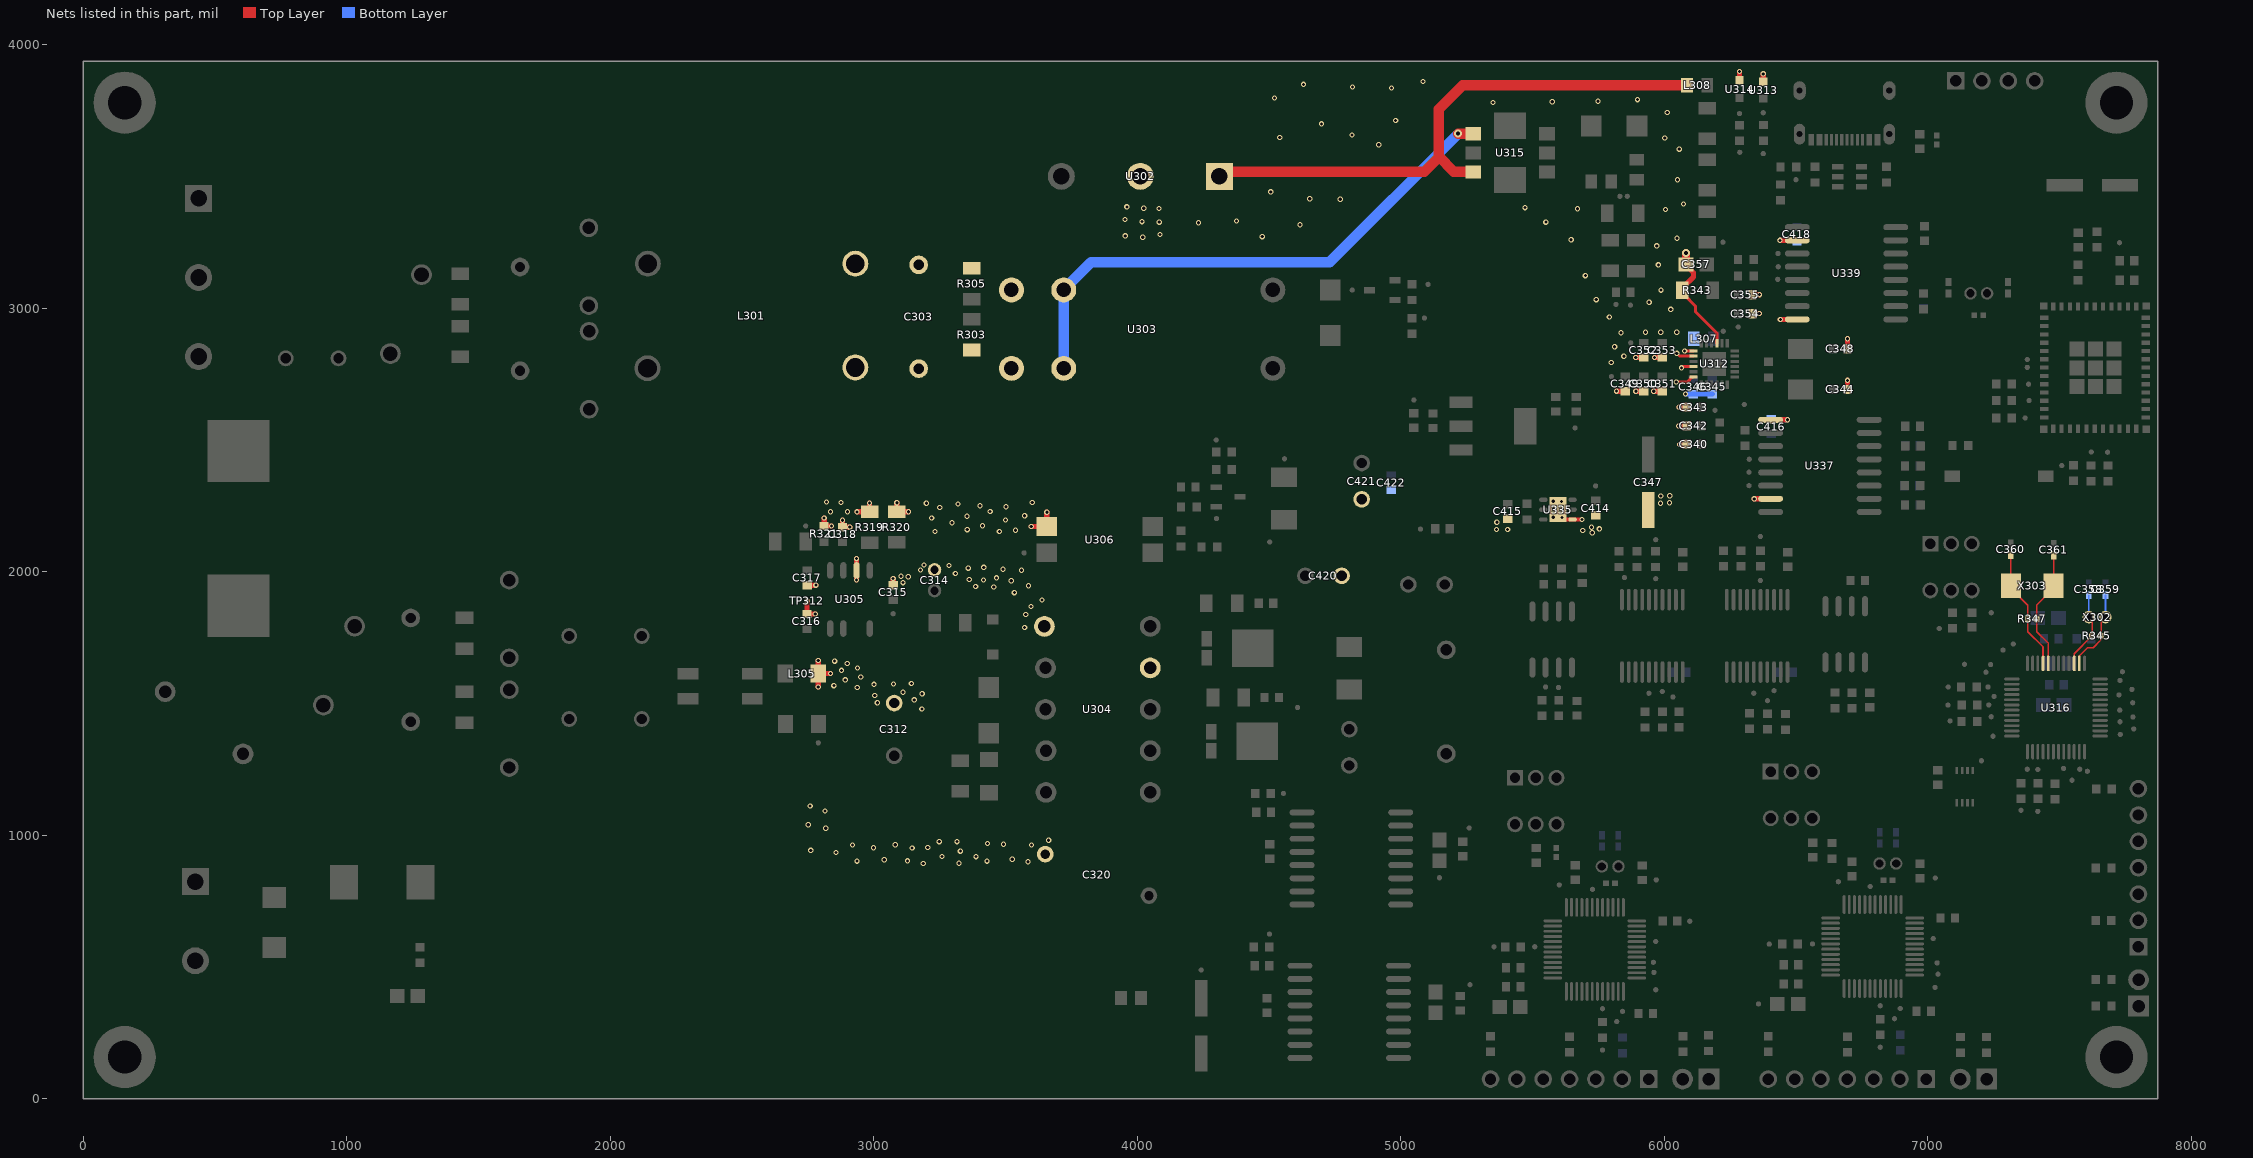
[diagram p0: the nets of this part, all layers, seen from the top]
# Altium PCB MISC84429.PcbDoc (part 2 of 5)
Units mil, origin at the board's own origin, x right, y up, seen from the top; angles counter-clockwise.
Board outline 7874.02 x 3937.01 mil, 4 copper layers (Top Layer, GND, POWER, Bottom Layer); 424 components, 202 nets, 1144 pads, 784 vias.

## Footprints (in the part's own frame and the unit in brackets; to place one, negate y for a bottom-side part, rotate by r counter-clockwise, add the part's x,y. Pads: shape width x height; smd on the part's side, far side on the other; paste and mask are expansions set on the pad) (continued)
CAP-TH_BD10.0-P5.00-D1.0-FD [mm]
  round 1.6 hole 1: 1(-2.54,0) 2(2.54,0)
  silkscreen extent -5,-5 5.08,5
CAP-TH_L7.0-W4.0-P10.00-D0.6 [mm]
  round 1.8 hole 1.1: 1(-5,0) 2(5,0)
  silkscreen extent -3.5,-2 3.5,2
CAP-TH_L8.0-W4.0-P7.50-D1.2 [mm]
  round 1.8 hole 1.2: 1(-3.75,0) 2(3.75,0)
  silkscreen extent -4,-2 4,2
CAP-TH_L10.0-W4.5-P10.00-D0.6-S4.0 [mm]
  round 1.6 hole 0.9: 1(-5,2) 2(5,-2)
  silkscreen extent -5,-2.25 5,2.25
CAP-TH_L13.0-W6.0-P10.00-D0.6 [mm]
  round 1.8 hole 1: 1(-5,0) 2(5,0)
  silkscreen extent -6.5,-3 6.5,3
CONN-TH_2P-P7.62_L15.2-W16.7-EX4.2 [mm]
  rect 2.6x2.6 hole 1.6: 1(-3.81,0)
  round 2.6 hole 1.6: 2(3.81,0)
  silkscreen extent -8.22,-10.65 8.38,4.55
CONN-TH_3P-P7.62_L15.2-W24.4-EX4.2 [mm]
  rect 2.6x2.6 hole 1.6: 1(-7.62,0)
  round 2.6 hole 1.6: 2(0,0) 3(7.62,0)
  silkscreen extent -12.03,-11 12.27,4.2
CRYSTAL-SMD_2P-L5.0-W3.2 [mm]
  rect 1.9x2.4 smd: 1(-1.95,0) 2(1.95,0)
  silkscreen extent -3.1,-1.75 3.1,1.75
CRYSTAL-SMD_L5.0-W3.2 [mm]
  rect 1.9x2.4 smd: 1(-2.05,0) 2(2.05,0)
  silkscreen extent -3.32,-1.85 3.33,1.85
F0603 [mil]
  rect 31.75x34.02 smd paste-3937.01 mask+2: 1(-29.66,0) 2(29.66,0)
  silkscreen extent -55,-25 55,25
FILTER-TH_FC-DLFW2015-5MH-20A-LF [mm]
  round 2.5 hole 1.8 paste+0 mask+0.05: 1(-5.04,-9.983) 2(5.04,-10.016) 3(4.96,10.016) 4(-5.04,10.016)
  silkscreen extent -13.72,-11.98 11.96,12.02
FUSE-SMD_L20.0-W5.0 [mm]
  rect 6x6 smd: 1(-7.45,0) 2(7.45,0)
  silkscreen extent -4.22,-2.58 4.17,2.55
FUSE-TH_L8.4-W4.0-P5.08-D0.6 [mil]
  round 60 hole 39.37 paste+0 mask+1.97: 1(-100,0) 2(100,0)
  silkscreen extent -170,-80 165,85
HDR-TH_2P-P2.54-V-M [mm]
  rect 2x2 hole 1.2: 1(-1.27,0)
  round 2 hole 1.2: 2(1.27,0)
  silkscreen extent -2.54,-1.27 2.54,1.27
HDR-TH_4P-P2.54-V-M [mm]
  rect 1.7x1.7 hole 1.1: 1(-3.81,0)
  round 1.7 hole 1.1: 2(-1.27,0) 3(1.27,0) 4(3.81,0)
  silkscreen extent -5.08,-1.27 5.08,1.27
HDR-TH_7P-P2.54-V-M [mm]
  rect 1.7x1.7 hole 1.1: 1(-7.62,0)
  round 1.7 hole 1.1: 2(-5.08,0) 3(-2.54,0) 4(0,0) 5(2.54,0) 6(5.08,0) 7(7.62,0)
  silkscreen extent -8.89,-1.25 8.89,1.25
IND-SMD_L5.4-W5.2_FXL0530 [mm]
  rect 1.9x2.5 smd: 1(-2.05,0) 2(2.05,0)
  silkscreen extent -2.7,-2.6 2.7,2.6
IND-TH_4P-L14.0-W12.0_DLSF1010-12MH-L-S [mm]
  round 1.524 hole 1 paste+0 mask+0.05: 1(-4,-3.5) 2(-4,3.5) 3(4,3.5) 4(4,-3.5)
  silkscreen extent -7.11,-5.97 6.98,6.1
L0805 [mil]
  rect 44.59x54.21 smd paste-3937.01 mask+2: 1(-38.04,0) 2(38.04,0)
  silkscreen extent -77,-40 73,40
L1206 [mm]
  rect 1.485x1.728 smd paste-100 mask+0.051: 1(-1.593,0) 2(1.593,0)
  silkscreen extent -2.56,-1.09 2.56,1.09
LED0603-R-FD [mm]
  rect 0.8x0.8 smd: 1(0.851,0) 2(-0.851,0)
  silkscreen extent -1.82,-0.86 1.77,0.86
LED0603-RD_GREEN [mm]
  rect 0.8x0.8 smd: 1(-0.799,-0.003) 2(0.799,0.003)
  silkscreen extent -1.49,-0.75 1.39,0.76
LQFP-48_L7.0-W7.0-P0.50-LS9.0-BL [mm]
  oval 0.27x1.5 smd paste+0 mask+0.05: 1(-2.75,-4.25) 2(-2.25,-4.25) 3(-1.75,-4.25) 4(-1.25,-4.25) 5(-0.75,-4.25) 6(-0.25,-4.25) 7(0.25,-4.25) 8(0.75,-4.25) 9(1.25,-4.25) 10(1.75,-4.25) 11(2.25,-4.25) 12(2.75,-4.25) 25(2.75,4.25) 26(2.25,4.25) 27(1.75,4.25) 28(1.25,4.25) 29(0.75,4.25) 30(0.25,4.25) 31(-0.25,4.25) 32(-0.75,4.25) 33(-1.25,4.25) 34(-1.75,4.25) 35(-2.25,4.25) 36(-2.75,4.25)
  oval 1.5x0.27 smd paste+0 mask+0.05: 13(4.25,-2.75) 14(4.25,-2.25) 15(4.25,-1.75) 16(4.25,-1.25) 17(4.25,-0.75) 18(4.25,-0.25) 19(4.25,0.25) 20(4.25,0.75) 21(4.25,1.25) 22(4.25,1.75) 23(4.25,2.25) 24(4.25,2.75) 37(-4.25,2.75) 38(-4.25,2.25) 39(-4.25,1.75) 40(-4.25,1.25) 41(-4.25,0.75) 42(-4.25,0.25) 43(-4.25,-0.25) 44(-4.25,-0.75) 45(-4.25,-1.25) 46(-4.25,-1.75) 47(-4.25,-2.25) 48(-4.25,-2.75)
  silkscreen extent -3.59,-4.46 3.3,3.34
LQFP-48_L7.0-W7.0-P0.50-LS9.0-TL [mm]
  oval 1.8x0.28 smd: 1(-4.05,2.75) 2(-4.05,2.25) 3(-4.05,1.75) 4(-4.05,1.25) 5(-4.05,0.75) 6(-4.05,0.25) 7(-4.05,-0.25) 8(-4.05,-0.75) 9(-4.05,-1.25) 10(-4.05,-1.75) 11(-4.05,-2.25) 12(-4.05,-2.75) 25(4.05,-2.75) 26(4.05,-2.25) 27(4.05,-1.75) 28(4.05,-1.25) 29(4.05,-0.75) 30(4.05,-0.25) 31(4.05,0.25) 32(4.05,0.75) 33(4.05,1.25) 34(4.05,1.75) 35(4.05,2.25) 36(4.05,2.75)
  oval 0.28x1.8 smd: 13(-2.75,-4.05) 14(-2.25,-4.05) 15(-1.75,-4.05) 16(-1.25,-4.05) 17(-0.75,-4.05) 18(-0.25,-4.05) 19(0.25,-4.05) 20(0.75,-4.05) 21(1.25,-4.05) 22(1.75,-4.05) 23(2.25,-4.05) 24(2.75,-4.05) 37(2.75,4.05) 38(2.25,4.05) 39(1.75,4.05) 40(1.25,4.05) 41(0.75,4.05) 42(0.25,4.05) 43(-0.25,4.05) 44(-0.75,4.05) 45(-1.25,4.05) 46(-1.75,4.05) 47(-2.25,4.05) 48(-2.75,4.05)
  silkscreen extent -4.42,-2.75 2.75,3.6
MBS_L4.7-W3.8-P2.40-LS7.0-TL [mm]
  rect 2x1.1 smd: 1(-3.1,1.2) 2(-3.1,-1.2) 3(3.1,-1.2) 4(3.1,1.2)
  silkscreen extent -3.23,-2.5 2.1,2.5
OSC-TH_BD3.1-P0.8-D0.3 [mm]
  round 1.2 hole 0.8: 1(0,0.8) 2(0,-0.8)
  silkscreen extent -10,-1.5 -0.7,1.5
R0402 [mm]
  rect 0.566x0.54 smd paste-100 mask+0.051: 1(-0.433,0) 2(0.433,0)
  silkscreen extent -0.94,-0.5 0.94,0.5
R0603 [mil]
  rect 31.75x34.02 smd paste-3937.01 mask+2: 1(-29.66,0) 2(29.66,0)
  silkscreen extent -55,-26 55,26
R1206 [mil]
  rect 47.54x66.97 smd paste-3937.01 mask+2: 1(-58.22,0) 2(58.22,0)
  silkscreen extent -91,-42 91,42
RELAY-TH_HF115F-XXX-1HS3 [mm]
  round 2.4 hole 1.4 paste+0 mask+0.05: 1(-12.6,3.78) 2(-12.6,-3.78) 5(7.56,3.78) 6(7.56,-3.78) 7(12.6,3.78) 8(12.6,-3.78)
  silkscreen extent -15.24,-6.35 13.84,6.35
RES-TH_L16.5-W5.6-P7.50-D1.2-S3.00 [mm]
  round 2 hole 1.4: 1(-3.8,1.5) 2(3.8,-1.5)
  silkscreen extent -8.25,-2.8 8.25,2.8
RES-TH_L17.5-W6.0-P7.50-D0.8-S7.50 [mm]
  round 2 hole 1.2 paste+0 mask+0.05: 1(-3.749,3) 2(3.749,-3)
  silkscreen extent -8.75,-3 8.75,3
SENSOR-TH_PA1005.100NL [mm]
  rect 1.27x1.52 smd: 1(1.85,3.555) 2(0,3.555) 3(-1.85,3.555) 4(-1.85,-3.555) 5(0,-3.555) 6(1.85,-3.555)
  rect 2.54x3.05 smd: 7(-2.615,0) 8(2.615,0)
  silkscreen extent -3.61,-4.19 3.6,4.19
SMA_L4.3-W2.6-LS5.2-RD [mm]
  rect 2x2 smd: 1(-2.2,0) 2(2.2,0)
  silkscreen extent -2.98,-1.5 2.6,1.5
SMB_L4.6-W3.6-LS5.4-RD [mil]
  rect 80.61x88.23 smd: 1(-95,0) 2(95,0)
  silkscreen extent -100,-77 88,77
SMC_L6.9-W5.9-LS7.9-RD [mm]
  rect 2.7x3.3 smd: 1(-3.686,0) 2(3.686,0)
  silkscreen extent -4.36,-3.1 3.98,3.1
SOD-123_L2.8-W1.8-LS3.7-RD [mm]
  rect 0.95x1.15 smd: 1(-1.692,0) 2(1.692,0)
  silkscreen extent -1.58,-0.87 1.41,0.87
SOIC-8_7P-L4.9-W3.9-P1.27-LS6.0-BL-PE3 [mm]
  oval 0.6x1.6 smd: 1(-1.905,-2.8) 2(-0.635,-2.8) 4(1.905,-2.8) 5(1.905,2.8) 6(0.635,2.8) 7(-0.635,2.8) 8(-1.905,2.8)
  silkscreen extent -2.54,-1.78 2.46,1.78
SOIC-8_L5.0-W4.0-P1.27-LS6.1-BL [mil]
  oval 22.38x76.78 smd: 1(-75,-106.5) 2(-25,-106.5) 3(25,-106.5) 4(75,-106.5) 5(75,106.5) 6(25,106.5) 7(-25,106.5) 8(-75,106.5)
  silkscreen extent -98,-58 98,58
SOIC-16_L10.3-W7.5-P1.27-LS10.3-BL [mil]
  oval 22.6x94.51 smd: 1(-175,-187.02) 2(-125,-187.02) 3(-75,-187.02) 4(-25,-187.02) 5(25,-187.02) 6(75,-187.02) 7(125,-187.02) 8(175,-187.02) 9(175,187.02) 10(125,187.02) 11(75,187.02) 12(25,187.02) 13(-25,187.02) 14(-75,187.02) 15(-125,187.02) 16(-175,187.02)
  silkscreen extent -210,-193 206,131
SOP-4_L6.5-W4.6-P2.54-LS10.2-TL [mm]
  rect 2x1.8 smd: 1(-5.1,1.27) 2(-5.1,-1.27) 3(5.1,-1.27) 4(5.1,1.27)
  silkscreen extent -4.42,-2.29 3.32,3.79
SOT-23-3_L2.9-W1.4-P1.91-LS2.6-BR [mm]
  rect 1.07x0.532 smd: 1(1.135,-0.955) 2(1.135,0.955) 3(-1.135,0)
  silkscreen extent -0.88,-1.54 0.88,1.54
SOT-23-3_L2.9-W1.6-P1.90-LS2.8-BR [mm]
  rect 1.07x0.6 smd: 1(1.235,-0.95) 2(1.235,0.95) 3(-1.235,0)
  silkscreen extent -0.88,-1.54 0.88,1.54
SOT-23-6_L2.9-W1.6-P0.95-LS2.8-BL [mil]
  rect 20.95x42.2 smd: 1(-37.4,-45.24) 2(0,-45.24) 3(37.4,-45.24) 4(37.4,45.24) 5(0,45.24) 6(-37.4,45.24)
  silkscreen extent -72,-57 61,35
SOT-223_L6.7-W3.5-P2.30-BR [mm]
  rect 2.2x1.1 smd: 1(3.099,-2.3) 2(3.099,0) 3(3.099,2.3)
  rect 2.2x3.5 smd: 4(-3.099,0)
  silkscreen extent -1.8,-3.55 1.8,3.55
SSOP-20_L7.2-W5.3-P0.65-LS7.8-BL [mil]
  oval 14.33x81.97 smd: 1(-115.16,-137.44) 2(-89.57,-137.44) 3(-63.98,-137.44) 4(-38.39,-137.44) 5(-12.79,-137.44) 6(12.8,-137.44) 7(38.39,-137.44) 8(63.98,-137.44) 9(89.57,-137.44) 10(115.16,-137.44) 11(115.16,137.44) 12(89.57,137.44) 13(63.98,137.44) 14(38.39,137.44) 15(12.8,137.44) 16(-12.79,137.44) 17(-38.39,137.44) 18(-63.98,137.44) 19(-89.57,137.44) 20(-115.16,137.44)
  silkscreen extent -146,-143 145,87
SW-SMD_2P-L3.5-W6.1-P2.54-LS9.8 [mm]
  rect 1.5x1.1 smd: 1(-4.5,0) 2(4.5,0)
  silkscreen extent -3.1,-1.27 3.1,1.27
SW-TH_5.8ZSGT [mm]
  rect 1.524x1.524 hole 1: 1(2,-2.25)
  round 1.524 hole 1: 2(0,-2.25) 3(-2,-2.25) 4(2,2.25) 5(0,2.25) 6(-2,2.25)
  silkscreen extent -3.05,-3.64 3.05,3.05
Test-Point-0.5mm [mm]
  round 0.5 smd: 1(0,0)
TO-277A_L4.7-W6.1-LS6.6-TR [mm]
  rect 1x1.5 smd: 1(2.21,0.9) 2(2.21,-0.9)
  rect 4x3.6 smd: 3(-2.21,0)
  silkscreen extent -3.84,-2.23 2.22,2.23
USB-C-SMD_TYPE-C-6PIN-2MD-073 [mm]
  rect 0.55x1.1 smd paste-100 mask+0.05: 1(-3.2,2.375) 2(-2.4,2.375) 11(2.4,2.375) 12(3.2,2.375)
  rect 0.3x1.1 smd paste-100 mask+0.05: 3(-1.75,2.375) 4(-1.25,2.375) 5(-0.75,2.375) 6(-0.25,2.375) 7(0.25,2.375) 8(0.75,2.375) 9(1.25,2.375) 10(1.75,2.375)
  oval 1.2x1.8 hole 0.6 slot 1.2 at 90 deg paste+0 mask+0.05: 13(-4.325,-2.375) 14(4.325,-2.375)
  oval 1.1x2 hole 0.6 slot 1.5 at 90 deg paste+0 mask+0.05: 13(-4.325,1.825) 14(4.325,1.825)
  Keep-Out Layer circle w0.005: c-2.89,1.305 r0.35
  Keep-Out Layer circle w0.005: c2.89,1.305 r0.35
  Keep-Out Layer board cut-out: 3.24,1.305 3.205,1.153 3.108,1.031 2.968,0.964 2.812,0.964 2.672,1.031 2.575,1.153 2.54,1.305 2.54,1.305 2.575,1.457 2.672,1.579 2.812,1.646 2.968,1.646 3.108,1.579 3.205,1.457 3.24,1.305
  Keep-Out Layer board cut-out: -2.54,1.305 -2.575,1.153 -2.672,1.031 -2.812,0.964 -2.968,0.964 -3.108,1.031 -3.205,1.153 -3.24,1.305 -3.24,1.305 -3.205,1.457 -3.108,1.579 -2.968,1.646 -2.812,1.646 -2.672,1.579 -2.575,1.457 -2.54,1.305
  Keep-Out Layer region: 3.24,1.305 3.205,1.153 3.108,1.031 2.968,0.964 2.812,0.964 2.672,1.031 2.575,1.153 2.54,1.305 2.54,1.305 2.575,1.457 2.672,1.579 2.812,1.646 2.968,1.646 3.108,1.579 3.205,1.457 3.24,1.305
  Keep-Out Layer region: -2.54,1.305 -2.575,1.153 -2.672,1.031 -2.812,0.964 -2.968,0.964 -3.108,1.031 -3.205,1.153 -3.24,1.305 -3.24,1.305 -3.205,1.457 -3.108,1.579 -2.968,1.646 -2.812,1.646 -2.672,1.579 -2.575,1.457 -2.54,1.305
  silkscreen extent -4.5,-4.97 4.57,0.6
VQFN-24_L4.0-W4.0-P0.50-BL-EP2.3 [mm]
  rect 0.3x0.8 smd paste-100 mask+0.051: 1(-1.25,-1.992) 2(-0.75,-1.991) 3(-0.25,-1.991) 4(0.25,-1.991) 5(0.75,-1.991) 6(1.25,-1.991) 13(1.25,1.992) 14(0.75,1.992) 15(0.25,1.992) 16(-0.25,1.992) 17(-0.75,1.992) 18(-1.25,1.992)
  rect 0.8x0.3 smd paste-100 mask+0.051: 7(1.998,-1.25) 8(1.998,-0.75) 9(1.998,-0.25) 10(1.998,0.25) 11(1.998,0.75) 12(1.998,1.25) 19(-1.998,1.25) 20(-1.998,0.75) 21(-1.998,0.25) 22(-1.998,-0.25) 23(-1.998,-0.75) 24(-1.998,-1.25)
  rect 2.3x2.3 smd paste-100 mask+0.051: 25(0.001,-0.001)
  silkscreen extent -2.1,-2.67 2.1,2.1
VSON8_L2.0-W2.3-P0.50-LS3.1-BL [mil]
  rect 9.84x27.56 smd: 1(-30,-61.03) 2(-10,-61.03) 3(10,-61.03) 4(30,-61.03) 5(30,61.03) 6(10,61.03) 7(-10,61.03) 8(-30,61.03)
  silkscreen extent -54,-74 47,39
VSON-6_L3.0-W3.0-P0.95-TL-EP_TI_DRP [mm]
  oval 0.817x0.427 smd: 1(-1.407,0.95) 2(-1.407,0) 3(-1.407,-0.95) 4(1.407,-0.95) 5(1.407,0) 6(1.407,0.95)
  rect 1.65x2.4 smd: 7(0,0)
  silkscreen extent -2.13,-1.58 1.58,1.58
WIFIM-SMD_61P-L16.6-W13.2-P0.80-ESP32-C6-MINI-1-N4 [mm]
  rect 0.8x0.4 smd paste+0 mask+0.05: 1(-5.9,3.975) 2(-5.9,3.175) 3(-5.9,2.375) 4(-5.9,1.575) 5(-5.9,0.775) 6(-5.9,-0.025) 7(-5.9,-0.825) 8(-5.9,-1.625) 9(-5.9,-2.425) 10(-5.9,-3.225) 11(-5.9,-4.025) 25(5.9,-4.025) 26(5.9,-3.225) 27(5.9,-2.425) 28(5.9,-1.625) 29(5.9,-0.825) 30(5.9,-0.025) 31(5.9,0.775) 32(5.9,1.575) 33(5.9,2.375) 34(5.9,3.175) 35(5.9,3.975)
  rect 0.4x0.8 smd paste+0 mask+0.05: 12(-4.8,-4.9) 13(-4,-4.9) 14(-3.2,-4.9) 15(-2.4,-4.9) 16(-1.6,-4.9) 17(-0.8,-4.9) 18(0,-4.9) 19(0.8,-4.9) 20(1.6,-4.9) 21(2.4,-4.9) 22(3.2,-4.9) 23(4,-4.9) 24(4.8,-4.9) 36(4.8,4.9) 37(4,4.9) 38(3.2,4.9) 39(2.4,4.9) 40(1.6,4.9) 41(0.8,4.9) 42(0,4.9) 43(-0.8,4.9) 44(-1.6,4.9) 45(-2.4,4.9) 46(-3.2,4.9) 47(-4,4.9) 48(-4.8,4.9)
  rect 1.45x1.45 smd paste+0 mask+0.05: 49(-1.775,1.85) 49(-1.775,0.05) 49(-1.775,-1.75) 49(0.025,1.85) 49(0.025,0.05) 49(0.025,-1.75) 49(1.825,1.85) 49(1.825,0.05) 49(1.825,-1.75)
  rect 0.7x0.7 smd paste+0 mask+0.05: 50(5.95,4.95) 51(5.95,-4.95) 52(-5.95,-4.95) 53(-5.95,4.95)
  silkscreen extent -7.57,-5.62 6.6,10.98

## Part data
C321 C325 C331 C366 C367 C368 C375 C385: library part GRM21BR61C106KE15L
C322: library part RVT100UF16V67RV0016
C323 C329: library part GRM188R61C226ME01D
C324 C330 C333 C335 C363 C364 C365 C371 C372 C373 C374 C381 C382 C383 C384 C389 C390 C391 C392 C393 C394 C395 C396 C397 C416 C417 C418 C419: library part GRM188R71E104KA01D
C326 C327 C362 C378 C388: library part GCM188R71C105KA64D
C328: library part Q07B1D101KN0B0N0N0
C332: library part GRM188R61E225KA12D
C334 C377 C414: library part GRM188R61E475KE11D
C358 C359 C369 C370 C379 C380: library part GJM1555C1H150FB01D
C360 C361: library part GJM1555C1H300FB01D
C376 C386: library part GRM1885C1H102JA01D
C387: library part GRT188C81E475KE13D
C415: library part CGA0603X5R105K500JT
D306: library part SS34_C154551
D307: library part SMBJ5.0A_C19077558
L303 L305: library part FCM3216KF-500T05
L307 L308 L309 L310: library part BLM21BD152SN1D
R301 R303 R304 R305 R308 R311: library part RC1206FR-07470KL
R306 R315: library part RC0603FR-071KL
R307 R355 R362 R370: library part RC0603FR-07100KL
R309 R432: library part RC1206FR-0722RL
R313: library part RC1206FR-07150KL
R314: library part RC1206JR-0710RL
R316: library part RK73H1JTTD2001F
R317: library part 1206W4F1025T5E
R318 R322 R323 R324 R325 R326 R327 R329 R331 R332 R354 R356 R357 R358 R359 R363 R365 R366 R367 R368 R371 R375 R376 R377 R390 R391 R392 R394 R400 R404 R405: library part RC0603FR-0710KL
R319 R320: library part RC1206FR-073R3L
R321: library part RC0603FR-0791KL
R328 R346 R348 R349 R350 R351 R352 R353 R361 R364 R372 R373 R378 R379 R380 R381 R382 R383 R384 R385 R386 R387 R388 R389 R393 R395 R403: library part FRC0603F33R0TS
R330 R337: library part RC0603FR-07100RL
R333: library part FRC0603F1004TS
R334 R335: library part RC0603FR-07160RL
R336: library part RC0603FR-0722KL
R338 R344: library part FRC1206F1001TS
R339 R340 R341: library part FRC1206F2703TS
R342: library part PA1206FRF470R05L
R343: library part RC1206JR-07470RL
R345 R360 R369 R374 R402: library part 0402WGF1002TCE
R347 R409: library part 0402WGF1004TCE
R396 R397 R398 R399 R407: library part RC0603FR-074K7L
R401: library part RC0603FR-070RL
R406 R408: library part RC0603FR-075K1L
R416: library part 0603WAF1002T5E
TP301 TP302 TP303 TP304 TP305 TP306 TP307 TP308 TP309 TP310 TP311 TP312 TP313 TP314 TP315 TP316 TP317 TP318 TP319 TP320 TP321 TP322 TP323 TP324 TP325 TP326 TP327 TP328 TP329 TP330 TP331 TP332 TP333 TP334 TP335 TP336 TP337 TP338 TP339 TP340 TP341 TP342 TP343 TP344 TP345 TP346 TP347 TP348 TP349 TP350 TP351 TP352 TP353 TP354 TP355 TP356 TP357 TP358 TP359 TP360 TP361 TP362 TP363 TP364 TP365 TP366 TP367 TP368 TP369 TP370 TP371 TP372 TP373 TP374 TP375 TP376 TP377 TP378 TP379 TP380 TP381 TP382 TP383 TP384 TP385 TP386 TP387 TP388 TP389 TP390 TP391 TP392 TP393 TP394 TP395 TP396 TP397 TP398 TP399 TP400 TP401 TP402 TP403 TP404 TP405 TP406 TP407 TP408 TP409 TP410 TP411 TP412 TP413 TP414 TP415 TP416 TP417 TP418 TP419 TP420 TP421 TP422 TP423 TP424 TP425 TP426 TP427 TP428 TP429: library part Test-Point
U304: library part EE19
U335: library part LDL212PU50R
X302 X304 X305: library part X308032768KGB2SC
X303: library part X50328MSB2GI

## Free pads (board coordinates)
  round 236.22 hole 125.98: 0(157.48,157.48) 1(7716.54,157.48) 2(7716.54,3779.53) 3(157.48,3779.53)

## Via types
v1: diameter 20, hole 12, Top Layer to Bottom Layer, tented both sides, 695 vias
v2: diameter 20, hole 12, Top Layer to Bottom Layer, 87 vias
v3: diameter 30, hole 15, Top Layer to Bottom Layer, tented both sides, 2 vias

## Nets (pads, with @x,y where several pads share a name; then routed paths per layer and width w, separated by ;. In a path a pad name is that pad's centre, name@x,y a point inside that pad or via, vN(x,y) a via of type N, cw(c..) or ccw(c..) an arc to the next point about the centre after c; other vN are vias at no path point)
220V_N_OUT: C303.1 C340.2 C342.2 C343.1 C344.1 C345.2 C346.2 C347.2 C348.1 C349.1 C350.1 C351.1 C352.1 C353.1 C354.1 C355.1 C357.1 C414.1 C415.1 C416.2 C418.2 C420.2 C421.2 C422.1 L301.4 L307.2 R305.1 R343.1 U302.2 U304.9 U312.9 U312.13 U312.14 U312.16 U312.18 U313.1 U314.2 U335.1 U335.7 U337.9 U337.15 U339.2 U339.8 | length 1586
  Top Layer w11: v1(6048,2828) 6058.47,2817.53 U312.14@6111.58,2817.53 ; v1(6077.78,2837.22) U312.13@6111.58,2837.22
  Top Layer w12: v2(6046,2719) 6087,2719 6106.79,2738.79 U312.18@6111.58,2738.79 ; v1(6066,2773) 6071.17,2778.17 U312.16@6111.58,2778.17 ; R343.1@6076,3050 6119,3007 6119,2986 6199.84,2905.16 U312.9@6199.84,2866.67
  Top Layer w16: U335.7@5621.6,2197.6 U335.1@5652.41,2197.6 v2(5688.6,2197.6)
  Top Layer w20: v1(5818.7,2684.7) C349.1@5852.28,2684.7 ; v1(5892.44,2812.44) C352.1@5923,2812.44 ; v1(5892.56,2684.44) C350.1@5922,2684.44 ; v1(5960.56,2684.44) C351.1@5993,2684.44 ; v1(5963.56,2812.44) C353.1@5993,2812.44 ; v1(6055.21,2552.79) C342.2@6085.42,2552.79 ; v1(6057,2624) C343.1@6085.44,2624 ; v1(6058.71,2482.54) C340.2@6085.42,2482.54 ; R343.1@6074,3081 6111,3118 6111,3134 6084.63,3160.37 C357.1@6084.63,3166 ; U314.2@6286,3864.5 v1(6286,3898) ; C354.1@6335.56,2979 v1(6360.72,2979) ; C355.1@6335.56,3051 v1(6361.72,3051) ; v2(6342,2276) U337.15@6403.98,2276 ; U313.1@6375.87,3858.47 v1(6375.87,3888.87) ; U337.9@6403.98,2576 v2(6468,2576) ; v2(6440,3257) U339.2@6504.98,3257 ; v2(6441,2957) U339.8@6504.98,2957 ; C344.1@6695.56,2691 v1(6695.56,2725.56) ; C348.1@6695.56,2846 v1(6695.56,2883.56)
  Top Layer w30: C357.1@6082.63,3166 v3(6082.63,3209.37)
  Bottom Layer w20: v1(6080.56,2673.44) C345.2@6183,2673.44 ; C416.2@6414,2576 v2(6468,2576) ; v2(6440,3257) C418.2@6493,3257
  Bottom Layer w40: U302.2@4016,3500 U302.2@4030,3500
  other v1: 5799,2793 5847,2817 5812,2853 5836,2906 5929,2908 5987,2908 6048,2908 5792,2966 6025,2995 5943,3022 5742,3032 5988,3068 5701,3123 5978,3164 5972,3236 5647,3259 6049,3265 4021,3269 4475,3271 3955,3274 4087,3279 4618,3316 4233,3324 4084,3326 5551,3326 4018,3328 4377,3330 3954,3336 6005,3374 5671,3377 4083,3378 4025,3379 5472,3381 3961,3384 6073,3395 4771,3413 4655,3415 4507,3441 6051,3487 6057,3603 4917,3620 6002,3645 4541,3647 4815,3657 4700,3699 4981,3712 6012,3742 5350,3780 5575,3783 5749,3785 5899,3791 4521,3797 4965,3835 4817,3839 4631,3849 5085,3860
  other v2: 5727,2147 5691,2156 5364,2160 5406,2160 5754,2162 5724,2168 5365,2187 5612,2205 5579,2206 5614,2237 5580,2238 5986,2259 6020,2261 5611,2266 5579,2267 5987,2287 6021,2288
220V_RELAY_IN: C303.2 L301.3 R303.2 U303.7 U303.8
220V_RELAY_OUT: U303.5 U303.6 U315.1 | length 2094.9
  Top Layer w40: v3(5218.17,3661.83) U315.1@5275.05,3661.83
  Bottom Layer w40: U303.5@3721.37,2771.19 3721.37,3070.37 3825,3174 4730,3174 v3@5216,3660
220V_TRANSFORMER_OUT: L308.1 U302.1 U315.3 | length 2158.4
  Top Layer w40: U302.1@4322,3496 4344,3518 5090,3518 5146,3574 ; U315.3@5263,3518 5202,3518 5144,3576 5144,3754 5236,3846 L308.1@6086.96,3846
AGND: C312.2 C314.2 C315.2 C316.1 C317.1 C318.1 C320.1 L305.2 R319.1 R320.1 R321.1 TP312.1 U304.1 U305.6 U306.3 | length 743.6
  Top Layer w20: C316.1@2747,1838.56 v1(2778.56,1838.56) ; C316.1@2747,1849 TP312.1@2747,1889 ; C317.1@2748,1948.44 v1(2780.56,1948.44) ; v1(2789.7,1562.3) L305.2@2789.7,1613 ; v1(2789.7,1662.7) L305.2@2789.7,1613 ; v1(2812,2203) R321.1@2812,2172.66 v1(2840.34,2172.66) ; v1(2836,1613) L305.2@2789.7,1613 ; v1(2882,2195) C318.1@2882,2168.56 v1(2909.56,2168.56) ; v1(2935,1968) U305.6@2935,2004.24 v1(2935,2049) ; v1(2936.44,2226.56) R319.1@2984.62,2226.56 v1(2984.62,2260.62) ; C315.2@3074,1948.56 v1(3074,1974) ; v1(3088,2261) R320.1@3088,2227.22 v1(3132.22,2227.22) ; v1(3598,2171) U306.3@3657.21,2171 v1(3657.21,2225.21)
  other v1: 3188,892 3324,893 3586,899 2937,901 3430,901 3128,902 3040,906 3526,908 3388,918 3259,919 2857,934 3329,939 2761,942 3146,951 2999,952 3205,953 2920,962 3599,962 3082,963 3493,965 3432,968 3249,975 3316,975 3664,980 2818,1026 2752,1039 2815,1091 2759,1110 3183,1478 3014,1502 3154,1513 3004,1530 3184,1536 3111,1542 2938,1560 2849,1567 3001,1572 3075,1573 3143,1575 2892,1589 2951,1600 2878,1625 2939,1634 2900,1651 2852,1660 3573,1788 3577,1837 3597,1867 3639,1892 3534,1920 3456,1941 3387,1943 3588,1946 3111,1958 3522,1965 3417,1968 3363,1970 3466,1976 3131,1980 3104,1982 3310,1993 3561,2005 3178,2006 3491,2009 3359,2013 3418,2016 3286,2023 3191,2025 3233,2152 3477,2152 3538,2157 3355,2159 3413,2174 3297,2185 3500,2196 3220,2203 3354,2210 3573,2212 2836,2227 2901,2227 3442,2228 3251,2243 3502,2246 3404,2250 3320,2256 3200,2259 2876,2262 3602,2262 2821,2264
CBT6_XTAL_8M_IN: C361.2 R347.1 U316.8 X303.1 | length 444
  Top Layer w6: U316.8@7457.47,1651.32 7457.47,1728.53 7414.04,1771.96 R347.1@7414.04,1820 7414.04,1873.04 X303.1@7477.71,1936.71 ; X303.1@7477.71,1947 C361.2@7477.71,2061.25
CBT6_XTAL_8M_OUT: C360.1 R347.2 U316.9 X303.2 | length 450
  Top Layer w6: X303.2@7316,1947.29 C360.1@7316,2062.54 ; X303.2@7316.29,1935.71 7379.96,1872.04 R347.2@7379.96,1820 7379.96,1772.04 7437.79,1714.21 U316.9@7437.79,1651.32
CBT6_XTAL_32.768KHZ_IN: C359.1 R345.1 U316.2 X302.1 | length 312
  Top Layer w6: U316.2@7575.58,1651.32 7575.58,1679.58 7607,1711 7628,1711 7658.04,1741.04 R345.1@7658.04,1756 7658.04,1810.54 X302.1@7674.5,1827
  Bottom Layer w6: X302.1@7675,1827.5 C359.1@7675,1910.54
CBT6_XTAL_32.768KHZ_OUT: C358.2 R345.2 U316.3 X302.2 | length 292.1
  Top Layer w6: U316.3@7555.9,1651.32 7555.9,1687.94 R345.2@7623.96,1756 7623.96,1814.54 X302.2@7611.5,1827
  Bottom Layer w6: X302.2@7612,1827.5 C358.2@7612,1910.54